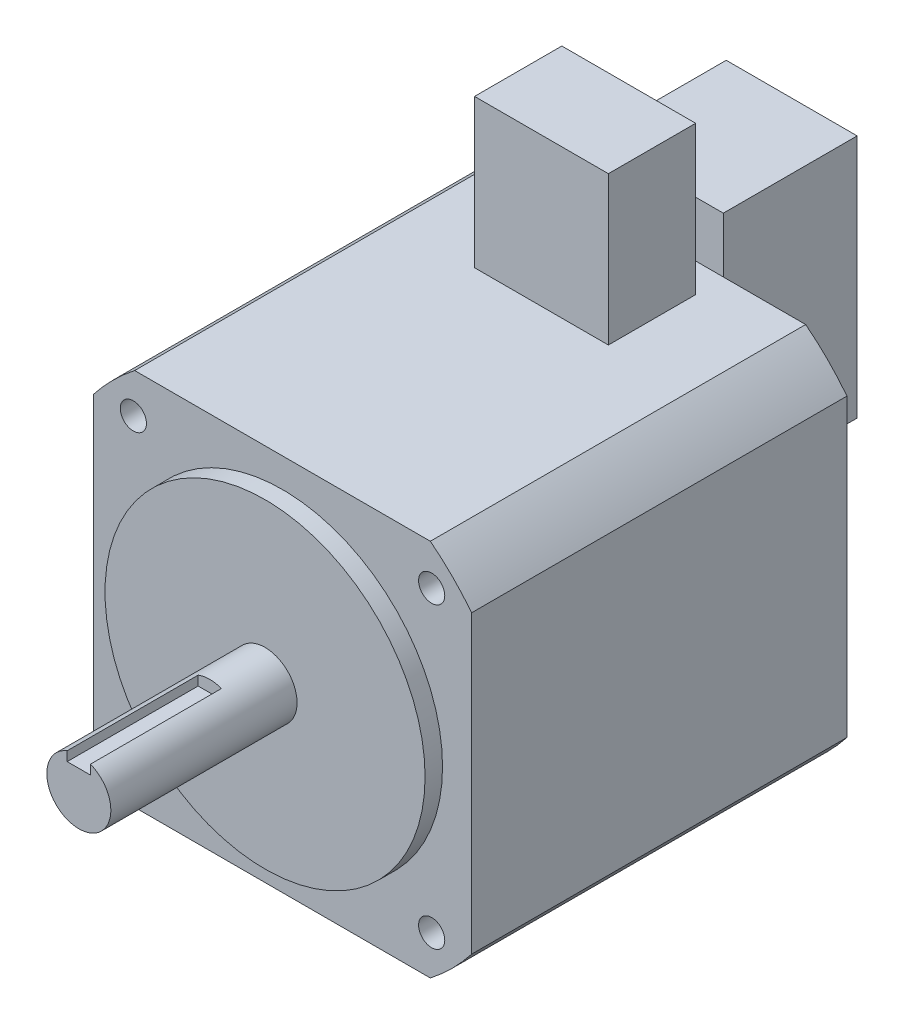
SolidWorks part; units mm, degrees
ref_plane "Front Plane" through (0, 0, 0) normal (0, 0, 1) x (1, 0, 0)
ref_plane "Top Plane" through (0, 0, 0) normal (0, 1, 0) x (1, 0, 0)
ref_plane "Right Plane" through (0, 0, 0) normal (1, 0, 0) x (0, 0, -1)
sketch "Sketch1" plane through (0, 0, 0) normal (0, 0, 1) x (1, 0, 0)
  line L1 (-65, 65) -> (65, 65)
  line L2 (-65, 65) -> (-65, -65)
  line L3 (-65, -65) -> (65, -65)
  line L4 (65, 65) -> (65, -65)
  line L5 (-65, 65) -> (65, -65) construction
  line L6 (-65, -65) -> (65, 65) construction
  point P0 (0, 0)
  dimension "D1" = 130
  dimension "D2" = 130
extrude "Boss-Extrude1" add sketch "Sketch1" along normal blind 12
sketch "Sketch2" plane through (0, 0, 12) normal (0, 0, 1) x (1, 0, 0)
  circle A0 centre (0, 0) radius 55
  dimension "D1" = 110
extrude "Boss-Extrude2" add sketch "Sketch2" along normal blind 6
sketch "Sketch3" plane through (0, 0, 18) normal (0, 0, 1) x (1, 0, 0)
  circle A0 centre (0, 0) radius 11
  dimension "D1" = 22
extrude "Boss-Extrude3" add sketch "Sketch3" along normal blind 64
sketch "Sketch4" plane through (0, 0, 12) normal (0, 0, 1) x (1, 0, 0)
  circle A0 centre (0, 0) radius 82.5
  dimension "D1" = 165
extrude "Cut-Extrude1" cut sketch "Sketch4" against normal blind 64 flip side to cut
hole_wizard "Ø9.0 (9) Diameter Hole1" positions "Sketch6" profile "Sketch5" hole size "Ø9.0" standard "GB"
sketch "Sketch6" plane through (0, 0, 12) normal (0, 0, 1) x (1, 0, 0)
  line L0 (-51.2652, 51.2652) -> (0, 0) construction
  line L2 (0, 72.5) -> (0, -72.5) construction
  circle A0 centre (0, 0) radius 72.5
  point P0 (-51.2652, 51.2652)
  dimension "D1" = 145
  dimension "D2" = 45
sketch "Sketch5" plane through (-51.2652, 51.2652, 12) normal (1, 0, 0) x (0, -1, 0)
  line L0 (0, 0) -> (0, 402.7039)
  line L1 (0, 402.7039) -> (4.5, 400)
  line L2 (4.5, 400) -> (4.5, 0)
  line L5 (4.5, 0) -> (0, 0)
  line L10 (0, 402.7039) -> (-4.5, 400) construction
  line L11 (0, -6.35) -> (0, 107.95) construction
  dimension "孔直径" = 9
  dimension "孔深度" = 400
  dimension "导头角度" = 118
pattern_circular "CirPattern1" count 4 over 360 about axis through (0, 0, 0) along (0, 0, 1) of "Ø9.0 (9) Diameter Hole1"
sketch "Sketch7" plane through (0, 0, 0) normal (0, 0, -1) x (-1, 0, 0)
  line L8 (-65, 50.806) -> (-65, -50.806)
  line L9 (-50.806, -65) -> (50.806, -65)
  line L10 (65, -50.806) -> (65, 50.806)
  line L11 (50.806, 65) -> (-50.806, 65)
  line L12 (-65, 50.806) -> (-65, -50.806)
  line L13 (-50.806, -65) -> (50.806, -65)
  line L14 (65, -50.806) -> (65, 50.806)
  line L15 (50.806, 65) -> (-50.806, 65)
  arc A8 (-50.806, 65) -> (-65, 50.806) centre (0, 0) ccw
  arc A9 (-65, -50.806) -> (-50.806, -65) centre (0, 0) ccw
  arc A10 (50.806, -65) -> (65, -50.806) centre (0, 0) ccw
  arc A11 (65, 50.806) -> (50.806, 65) centre (0, 0) ccw
  arc A12 (-50.806, 65) -> (-65, 50.806) centre (0, 0) ccw
  arc A13 (-65, -50.806) -> (-50.806, -65) centre (0, 0) ccw
  arc A14 (50.806, -65) -> (65, -50.806) centre (0, 0) ccw
  arc A15 (65, 50.806) -> (50.806, 65) centre (0, 0) ccw
  dimension "D1" = 0
extrude "Boss-Extrude4" add sketch "Sketch7" along normal blind 117
sketch "Sketch8" plane through (0, 0, -117) normal (0, 0, -1) x (-1, 0, 0)
  line L0 (0, 65) -> (0, -93.0096) construction
  line L1 (-22.5, 0) -> (22.5, 0)
  line L2 (-22.5, 0) -> (-22.5, 84)
  line L3 (-22.5, 84) -> (22.5, 84)
  line L4 (22.5, 0) -> (22.5, 84)
  line L5 (50.806, 65) -> (-50.806, 65) construction
  dimension "D1" = 45
  dimension "D2" = 84
extrude "Boss-Extrude5" add sketch "Sketch8" along normal blind 46
sketch "Sketch9" plane through (0, 0, 0) normal (1, 0, 0) x (0, 0, -1)
  line L0 (117, 65) -> (-12, 65) construction
  line L1 (107, 65) -> (77, 65)
  line L2 (107, 65) -> (107, 116)
  line L3 (107, 116) -> (77, 116)
  line L4 (77, 65) -> (77, 116)
  line L5 (117, 50.806) -> (117, 65) construction
  dimension "D1" = 116
  dimension "D2" = 10
  dimension "D3" = 30
extrude "Boss-Extrude6" add sketch "Sketch9" along normal mid plane 46
sketch "Sketch10" plane through (0, 0, 82) normal (0, 0, 1) x (1, 0, 0)
  line L1 (-4, 7) -> (4, 7)
  line L2 (-4, 7) -> (-4, 17)
  line L3 (-4, 17) -> (4, 17)
  line L4 (4, 7) -> (4, 17)
  line L5 (-4, 7) -> (4, 17) construction
  line L6 (-4, 17) -> (4, 7) construction
  circle A0 centre (0, 0) radius 11 construction
  point P0 (0, 12)
  dimension "D1" = 8
  dimension "D2" = 7
  dimension "D3" = 10
extrude "Cut-Extrude2" cut sketch "Sketch10" against normal blind 45
